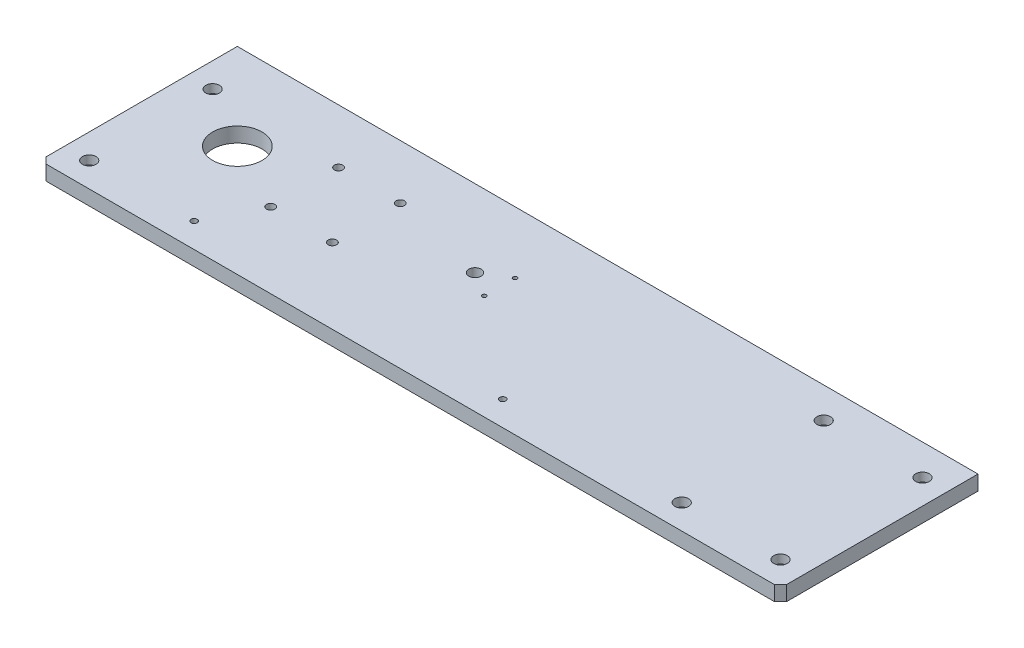
SolidWorks part; units mm, degrees
material "45#"
ref_plane "Front Plane" through (0, 0, 0) normal (0, 0, 1) x (1, 0, 0)
ref_plane "Top Plane" through (0, 0, 0) normal (0, 1, 0) x (1, 0, 0)
ref_plane "Right Plane" through (0, 0, 0) normal (1, 0, 0) x (0, 0, -1)
sketch "Sketch1" plane through (0, 0, 0) normal (0, 1, 0) x (1, 0, 0)
  line L0 (300, 80) -> (-300, -80) construction
  line L1 (-300, 80) -> (300, 80)
  line L2 (-300, 80) -> (-300, -80)
  line L3 (-300, -80) -> (300, -80)
  line L4 (300, 80) -> (300, -80)
  dimension "D1" = 600
  dimension "D2" = 160
extrude "Extrude1" add sketch "Sketch1" along normal mid plane 12
sketch "Sketch2" plane through (0, 6, 0) normal (0, 1, 0) x (1, 0, 0)
  point P0 (-280, 40)
  point P1 (-280, -60)
  point P3 (200, -60)
  point P5 (280, -60)
  point P7 (200, 55)
  point P9 (280, 55)
hole_wizard "M6 Socket Head Cap Screw Counterbore1" positions "3D Sketch1" profile "Sketch3" counterbore size "M6" standard "ISO" end condition through all
sketch3d "3D Sketch1"
  point P0 (-280, 6, 60)
  point P3 (-280, 6, -40)
  point P6 (200, 6, 60)
  point P9 (200, 6, -55)
  point P12 (280, 6, -55)
  point P15 (280, 6, 60)
sketch "Sketch3" plane through (-280, 6, 60) normal (1, 0, 0) x (0, 0, 1)
  line L0 (0, 0) -> (0, 12)
  line L1 (0, 12) -> (3.3, 12)
  line L3 (3.3, 12) -> (3.3, 7)
  line L4 (3.3, 7) -> (5.5, 7)
  line L5 (5.5, 7) -> (5.5, 0)
  line L7 (5.5, 0) -> (0, 0)
  line L11 (0, -6.35) -> (0, 107.95) construction
  dimension "貫穿孔直徑" = 6.6
  dimension "貫穿孔深度" = 12
  dimension "柱孔直徑" = 11
  dimension "柱孔深度" = 7
sketch "Sketch4" plane through (0, 0, -80) normal (0, 0, -1) x (-1, 0, 0)
  point P0 (230, 0)
  point P3 (-20, 0)
  point P7 (-270, 0)
hole_wizard "M4 Tapped Hole1" positions "3D Sketch2" profile "Sketch5" tap size "M4" standard "ISO"
sketch3d "3D Sketch2"
  point P0 (270, 0, -80)
  point P6 (20, 0, -80)
  point P12 (-230, 0, -80)
sketch "Sketch5" plane through (270, 0, -80) normal (1, 0, 0) x (0, 1, 0)
  line L0 (0, 0) -> (0, 11.0914)
  line L1 (0, 11.0914) -> (1.65, 10.1)
  line L2 (1.65, 10.1) -> (1.65, 0)
  line L5 (1.65, 0) -> (0, 0)
  line L10 (0, 11.0914) -> (-1.65, 10.1) construction
  line L11 (0, -6.35) -> (0, 107.95) construction
  dimension "螺孔鑽直徑" = 3.3
  dimension "螺孔鑽深度" = 10.1
  dimension "導頭角度" = 118
cosmetic thread "Cosmetic Thread1" parameters "D1"=8, "D2"=4
cosmetic thread "Cosmetic Thread2" parameters "D1"=8, "D2"=4
cosmetic thread "Cosmetic Thread3" parameters "D1"=8, "D2"=4
sketch "Sketch6" plane through (0, 6, 0) normal (0, 1, 0) x (1, 0, 0)
  line L0 (-174, -24) -> (-174, -14) construction
  line L2 (-174, 31) -> (-174, 41) construction
  line L4 (-124, 41) -> (-124, 31) construction
  line L6 (-124, -14) -> (-124, -24) construction
hole_wizard "M8 Tapped Hole1" positions "3D Sketch3" profile "Sketch7" tap size "M8" standard "ISO" end condition through all
sketch3d "3D Sketch3"
  line L1 (-174, 6, 24) -> (-174, 6, 14) construction
  line L2 (-124, 6, 14) -> (-124, 6, 24) construction
  line L3 (-124, 6, -41) -> (-124, 6, -31) construction
  line L4 (-174, 6, -31) -> (-174, 6, -41) construction
  point P4 (-174, 6, 19)
  point P6 (-124, 6, 19)
  point P8 (-124, 6, -36)
  point P10 (-174, 6, -36)
sketch "Sketch7" plane through (-174, 6, 19) normal (1, 0, 0) x (0, 0, 1)
  line L0 (0, 0) -> (0, 12)
  line L1 (0, 12) -> (3.4, 12)
  line L2 (3.4, 12) -> (3.4, 0)
  line L5 (3.4, 0) -> (0, 0)
  line L11 (0, -6.35) -> (0, 107.95) construction
  dimension "貫穿螺孔鑽直徑" = 6.8
  dimension "貫穿螺孔鑽深度" = 12
cosmetic thread "Cosmetic Thread6" parameters "D2"=8
cosmetic thread "Cosmetic Thread7" parameters "D2"=8
cosmetic thread "Cosmetic Thread8" parameters "D2"=8
cosmetic thread "Cosmetic Thread9" parameters "D2"=8
sketch "Sketch8" plane through (0, 6, 0) normal (0, 1, 0) x (1, 0, 0)
  point P0 (-195, -60)
  point P1 (55, -60)
hole_wizard "M6 Tapped Hole2" positions "3D Sketch4" profile "Sketch9" tap size "M6" standard "ISO" end condition through all
sketch3d "3D Sketch4"
  point P0 (55, 6, 60)
  point P3 (-195, 6, 60)
sketch "Sketch9" plane through (55, 6, 60) normal (1, 0, 0) x (0, 0, 1)
  line L0 (0, 0) -> (0, 12)
  line L1 (0, 12) -> (2.5, 12)
  line L2 (2.5, 12) -> (2.5, 0)
  line L5 (2.5, 0) -> (0, 0)
  line L11 (0, -6.35) -> (0, 107.95) construction
  dimension "貫穿螺孔鑽直徑" = 5
  dimension "貫穿螺孔鑽深度" = 12
cosmetic thread "Cosmetic Thread10" parameters "D2"=6
cosmetic thread "Cosmetic Thread11" parameters "D2"=6
sketch "Sketch10" plane through (0, 6, 0) normal (0, 1, 0) x (1, 0, 0)
  line L0 (300, 80) -> (-300, 80) construction
  line L1 (-300, 80) -> (-300, -80) construction
  circle A0 centre (-230, 10) radius 20
  dimension "D2" = 70
  dimension "D3" = 40
  dimension "D1" = 70
extrude "Cut-Extrude1" cut sketch "Sketch10" against normal through all
hole_wizard "M4 Tapped Hole2" positions "3D Sketch6" profile "Sketch12" tap size "M4" standard "ISO"
sketch3d "3D Sketch6"
  line L0 (-25, 6, -5) -> (-25, 6, -30) construction
  line L1 (-25, 6, -30) -> (-25, 6, -80) construction
  line L2 (300, 6, -80) -> (-300, 6, -80) construction
  line L4 (300, 6, 80) -> (300, 6, -80) construction
  point P0 (-25, 6, -5)
  point P2 (-25, 6, -30)
  dimension "D3" = 325
  dimension "D1" = 25
  dimension "D2" = 50
sketch "Sketch12" plane through (-25, 6, -5) normal (1, 0, 0) x (0, 0, 1)
  line L0 (0, 0) -> (0, 12.9914)
  line L1 (0, 12.9914) -> (1.65, 12)
  line L2 (1.65, 12) -> (1.65, 0)
  line L5 (1.65, 0) -> (0, 0)
  line L10 (0, 12.9914) -> (-1.65, 12) construction
  line L11 (0, -6.35) -> (0, 107.95) construction
  dimension "螺孔鑽直徑" = 3.3
  dimension "螺孔鑽深度" = 12
  dimension "導頭角度" = 118
cosmetic thread "Cosmetic Thread12" parameters "D1"=8, "D2"=4
cosmetic thread "Cosmetic Thread13" parameters "D1"=8, "D2"=4
chamfer "Chamfer1" distance 5 angle 45 2 edges at (-300, 0, 80) (300, 0, 80)
sketch "Sketch13" plane through (0, 6, 0) normal (0, 1, 0) x (1, 0, 0)
  line L0 (-25, 30) -> (-25, 5) construction
  line L1 (-45, 17.5) -> (-25, 17.5) construction
  circle A0 centre (-45, 17.5) radius 5
  dimension "D1" = 10
  dimension "D2" = 20
extrude "Cut-Extrude2" cut sketch "Sketch13" against normal through all
